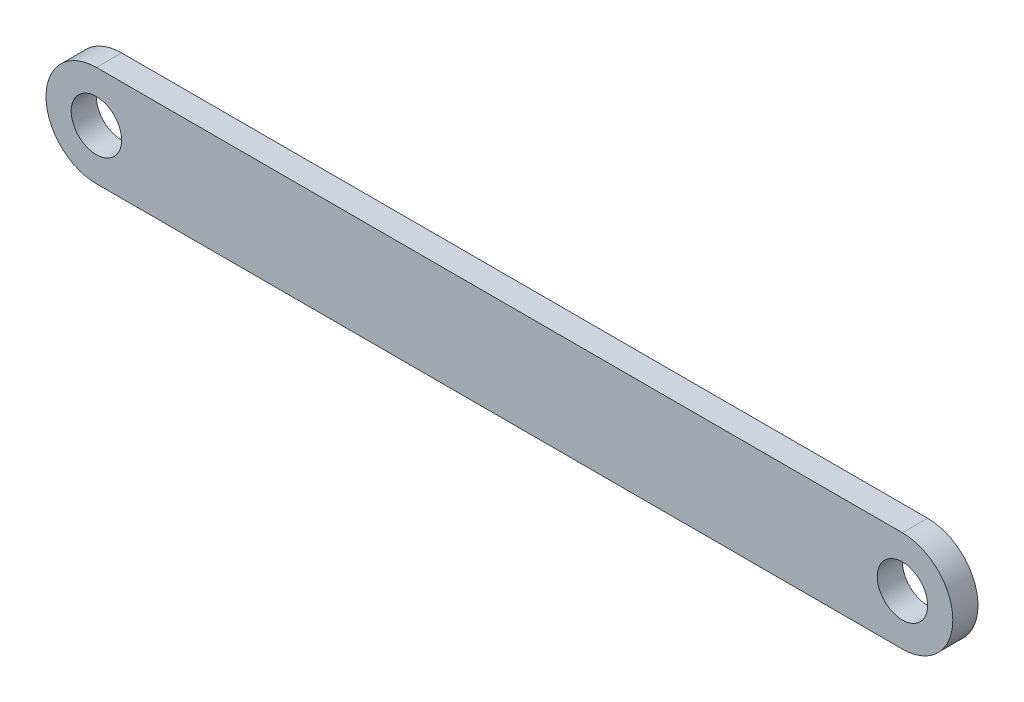
SolidWorks part; units mm, degrees
ref_plane "Front Plane" through (0, 0, 0) normal (0, 0, 1) x (1, 0, 0)
ref_plane "Top Plane" through (0, 0, 0) normal (0, 1, 0) x (1, 0, 0)
ref_plane "Right Plane" through (0, 0, 0) normal (1, 0, 0) x (0, 0, -1)
sketch "Sketch1" plane through (0, 0, 0) normal (0, 0, 1) x (1, 0, 0)
  line L0 (0, 0) -> (64, 0) construction
  line L1 (0, 4) -> (64, 4)
  line L2 (0, -4) -> (64, -4)
  arc A0 (0, 4) -> (0, -4) centre (0, 0) ccw
  arc A1 (64, -4) -> (64, 4) centre (64, 0) ccw
  circle A2 centre (0, 0) radius 2
  circle A3 centre (64, 0) radius 2
  point P3 (32, 0)
  dimension "D2" = 4
  dimension "D3" = 4
  dimension "D4" = 4
  dimension "D1" = 64
extrude "Boss-Extrude1" add sketch "Sketch1" along normal blind 2
